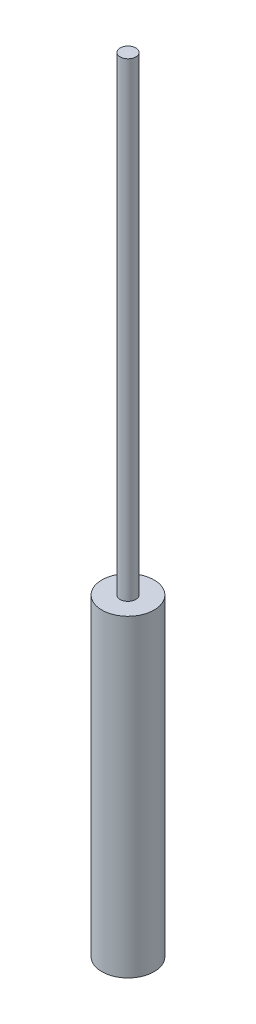
from build123d import *

# Parameters (mm, degrees)
SKETCH1_R                   = 5
BOSS_EXTRUDE1_DEPTH         = 60
SKETCH2_R                   = 1.5
BOSS_EXTRUDE2_DEPTH         = 90
M4_TAPPED_HOLE1_D           = 3.3
M4_TAPPED_HOLE1_DEPTH       = 11.5
M4_TAPPED_HOLE1_CSINK_D     = 4.05
M4_TAPPED_HOLE1_CSINK_ANGLE = 90
M4_TAPPED_HOLE1_TIP         = 0.991420021


with BuildPart() as part:
    # Sketch1 → Boss-Extrude1 (new body)
    with BuildSketch(Plane(origin=(0, 0, 0), x_dir=(1, 0, 0), z_dir=(0, 1, 0))):
        with Locations(Location((0, 0, 0), (0, 0, 270))):
            Circle(SKETCH1_R)
    extrude(amount=BOSS_EXTRUDE1_DEPTH)

    # Sketch2 → Boss-Extrude2 (add)
    with BuildSketch(Plane(origin=(0, 60, 0), x_dir=(1, 0, 0), z_dir=(0, 1, 0))):
        with Locations(Location((0, 0, 0), (0, 0, 90))):
            Circle(SKETCH2_R)
    extrude(amount=BOSS_EXTRUDE2_DEPTH)

    # M4 Tapped Hole1
    with Locations(Plane(origin=(0, 0, 0), x_dir=(-1, 0, 0), z_dir=(0, -1, 0))):
        with Locations((0, 0)):
            CounterSinkHole(M4_TAPPED_HOLE1_D / 2, M4_TAPPED_HOLE1_CSINK_D / 2, depth=M4_TAPPED_HOLE1_DEPTH, counter_sink_angle=M4_TAPPED_HOLE1_CSINK_ANGLE)
            with Locations((0, 0, -(M4_TAPPED_HOLE1_DEPTH + M4_TAPPED_HOLE1_TIP / 2))):  # 118° drill point
                Cone(0, M4_TAPPED_HOLE1_D / 2, M4_TAPPED_HOLE1_TIP, mode=Mode.SUBTRACT)


solid = part.part
